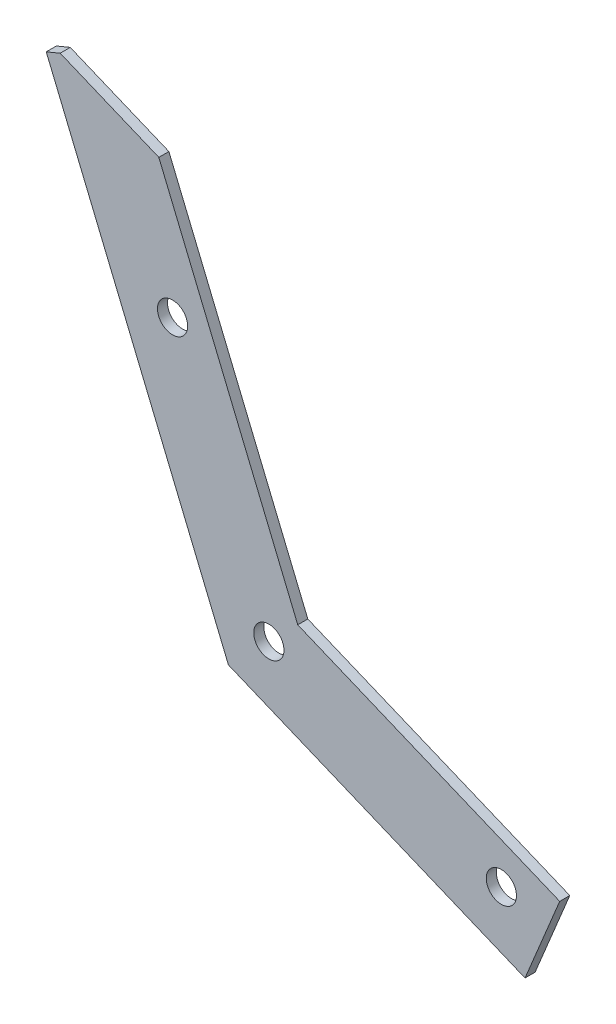
SolidWorks part; units mm, degrees
ref_plane "Front Plane" through (0, 0, 0) normal (0, 0, 1) x (1, 0, 0)
ref_plane "Top Plane" through (0, 0, 0) normal (0, 1, 0) x (1, 0, 0)
ref_plane "Right Plane" through (0, 0, 0) normal (1, 0, 0) x (0, 0, -1)
sketch "Sketch1" plane through (0, 0, 0) normal (0, 0, 1) x (1, 0, 0)
  line L0 (-174.2651, 0) -> (-123.2241, -123.2241)
  line L1 (0, -174.2651) -> (123.2241, -123.2241)
  line L2 (123.2241, -123.2241) -> (174.2651, 0)
  line L3 (174.2651, 0) -> (123.2241, 123.2241)
  line L4 (123.2241, 123.2241) -> (0, 174.2651)
  line L5 (0, 174.2651) -> (-123.2241, 123.2241)
  line L6 (-123.2241, 123.2241) -> (-174.2651, 0)
  line L7 (-123.2241, -123.2241) -> (0, -174.2651)
  circle A0 centre (0, 0) radius 161 construction
  dimension "D1" = 322
extrude "Boss-Extrude1" add sketch "Sketch1" along normal blind 310
shell "Shell1" thickness 2
sketch "Sketch2" plane through (0, 0, 310) normal (0, 0, 1) x (1, 0, 0)
  line L48 (104.0899, 104.0899) -> (0, 147.2053)
  line L49 (147.2053, 0) -> (104.0899, 104.0899)
  line L50 (104.0899, -104.0899) -> (147.2053, 0)
  line L51 (0, -147.2053) -> (104.0899, -104.0899)
  line L52 (-104.0899, -104.0899) -> (0, -147.2053)
  line L53 (-147.2053, 0) -> (-104.0899, -104.0899)
  line L54 (-104.0899, 104.0899) -> (-147.2053, 0)
  line L55 (0, 147.2053) -> (-104.0899, 104.0899)
  line L56 (104.0899, 104.0899) -> (0, 147.2053)
  line L57 (147.2053, 0) -> (104.0899, 104.0899)
  line L58 (104.0899, -104.0899) -> (147.2053, 0)
  line L59 (0, -147.2053) -> (104.0899, -104.0899)
  line L60 (-104.0899, -104.0899) -> (0, -147.2053)
  line L61 (-147.2053, 0) -> (-104.0899, -104.0899)
  line L62 (-104.0899, 104.0899) -> (-147.2053, 0)
  line L63 (0, 147.2053) -> (-104.0899, 104.0899)
  dimension "D1" = 25
extrude "Cut-Extrude1" cut sketch "Sketch2" against normal blind 10
sketch "Sketch3" plane through (0, 0, 310) normal (0, 0, 1) x (1, 0, 0)
  line L0 (0, 0) -> (19134.1716, 46193.9766) construction
  line L1 (104.0899, 104.0899) -> (0, 147.2053) construction
  line L2 (70.1382, 169.3285) -> (-63.801, -154.0293)
  line L3 (-63.801, -154.0293) -> (130.028, -234.3159)
  line L4 (130.028, -234.3159) -> (263.9672, 89.0419)
  line L5 (70.1382, 169.3285) -> (263.9672, 89.0419)
  point P5 (52.0449, 125.6476)
  dimension "D1" = 350
extrude "Cut-Extrude2" cut sketch "Sketch3" against normal through all
sketch "Sketch4" plane through (0, 0, 310) normal (0, 0, 1) x (1, 0, 0)
  line L0 (-122.414, 50.7056) -> (46071.5626, -19083.4661) construction
  line L1 (-104.0899, 104.0899) -> (-147.2053, 0) construction
  line L2 (-143.9329, 151.6223) -> (-51.5449, 113.354)
  line L3 (-208.9891, -5.4372) -> (-116.6011, -43.7056)
  line L4 (-51.5449, 113.354) -> (-116.6011, -43.7056)
  line L5 (-143.9329, 151.6223) -> (-208.9891, -5.4372)
  line L6 (-123.2241, 123.2241) -> (-174.2651, 0) construction
  point P4 (-125.6476, 52.0449)
  dimension "D1" = 170
  dimension "D2" = 100
  dimension "D3" = 30
extrude "Cut-Extrude3" cut sketch "Sketch4" against normal blind 5
sketch "Sketch5" plane through (0, 0, 310) normal (0, 0, 1) x (1, 0, 0)
  line L0 (0, 0) -> (-46193.9766, 19134.1716) construction
  line L1 (-114.805, 114.805) -> (-162.3588, 0) construction
  line L2 (-0.8258, 155.6653) -> (46193.1508, -18978.5063) construction
  line L3 (-82.5215, 121.1418) -> (46111.4551, 19255.3134) construction
  line L4 (0, 147.2053) -> (-66.6347, 119.6043) construction
  line L5 (52.0449, 125.6476) -> (0, 147.2053) construction
  circle A0 centre (0, 155.3233) radius 3
  circle A2 centre (-46.194, 136.1891) radius 3
  circle A3 centre (46.194, 136.1891) radius 3
  circle A4 centre (-128.9643, -63.6362) radius 3
  circle A6 centre (-109.8301, -109.8301) radius 3
  circle A7 centre (-63.6362, -128.9643) radius 3
  point P5 (-138.5819, 57.4025)
  dimension "D3" = 6
  dimension "D4" = 50
  dimension "D5" = 50
  dimension "D6" = 6
  dimension "D1" = 7.5
  dimension "D2" = 7.5
extrude "Cut-Extrude4" cut sketch "Sketch5" against normal blind 10
sketch "Sketch19" plane through (0, 0, 310) normal (0, 0, 1) x (1, 0, 0)
  line L0 (-32.5281, -78.5298) -> (61.612, 148.7446)
  line L1 (61.612, 148.7446) -> (-87.1326, 210.3566)
  line L2 (-87.1326, 210.3566) -> (-181.2727, -16.9177)
  line L3 (-181.2727, -16.9177) -> (-32.5281, -78.5298)
  line L4 (-164.355, -23.9253) -> (-131.6909, -37.4552) construction
  line L5 (61.612, 148.7446) -> (0, 174.2651) construction
  line L6 (61.612, 148.7446) -> (52.0449, 125.6476) construction
  line L7 (-123.2241, 123.2241) -> (-174.2651, 0) construction
extrude "Cut-Extrude5" cut sketch "Sketch19" against normal through all
sketch "Sketch21" plane through (0, 0, 310) normal (0, 0, 1) x (1, 0, 0)
  line L2 (-164.355, -23.9253) -> (-123.2241, -123.2241) construction
  line L3 (-123.2241, -123.2241) -> (-61.612, -148.7446) construction
  line L4 (-117.8665, -117.8665) -> (-58.9332, -142.2774)
  line L5 (-148.3207, -44.3435) -> (-117.8665, -117.8665)
  line L6 (-117.8665, -117.8665) -> (-58.9332, -142.2774)
  line L7 (-155.209, -27.7137) -> (-117.8665, -117.8665)
  line L8 (-164.355, -23.9253) -> (-123.2241, -123.2241)
  line L9 (-123.2241, -123.2241) -> (-61.612, -148.7446)
  line L10 (-52.0449, -125.6476) -> (-61.612, -148.7446) construction
  line L11 (-164.355, -23.9253) -> (-131.6909, -37.4552) construction
  line L12 (-58.9332, -142.2774) -> (-61.612, -148.7446)
  line L13 (-164.355, -23.9253) -> (-155.209, -27.7137)
  dimension "D1" = 18
extrude "Cut-Extrude7" cut sketch "Sketch21" against normal through all
sketch "Sketch22" plane through (0, 0, 310) normal (0, 0, 1) x (1, 0, 0)
  line L0 (-117.8665, -117.8665) -> (-155.209, -27.7137) construction
  line L1 (-155.209, -27.7137) -> (-131.6909, -37.4552) construction
  line L2 (-154.061, -30.4853) -> (-155.209, -27.7137)
  line L3 (-155.209, -27.7137) -> (-151.2893, -29.3372)
  line L4 (-154.061, -30.4853) -> (-151.2893, -29.3372)
  dimension "D1" = 3
extrude "Cut-Extrude8" cut sketch "Sketch22" against normal through all
